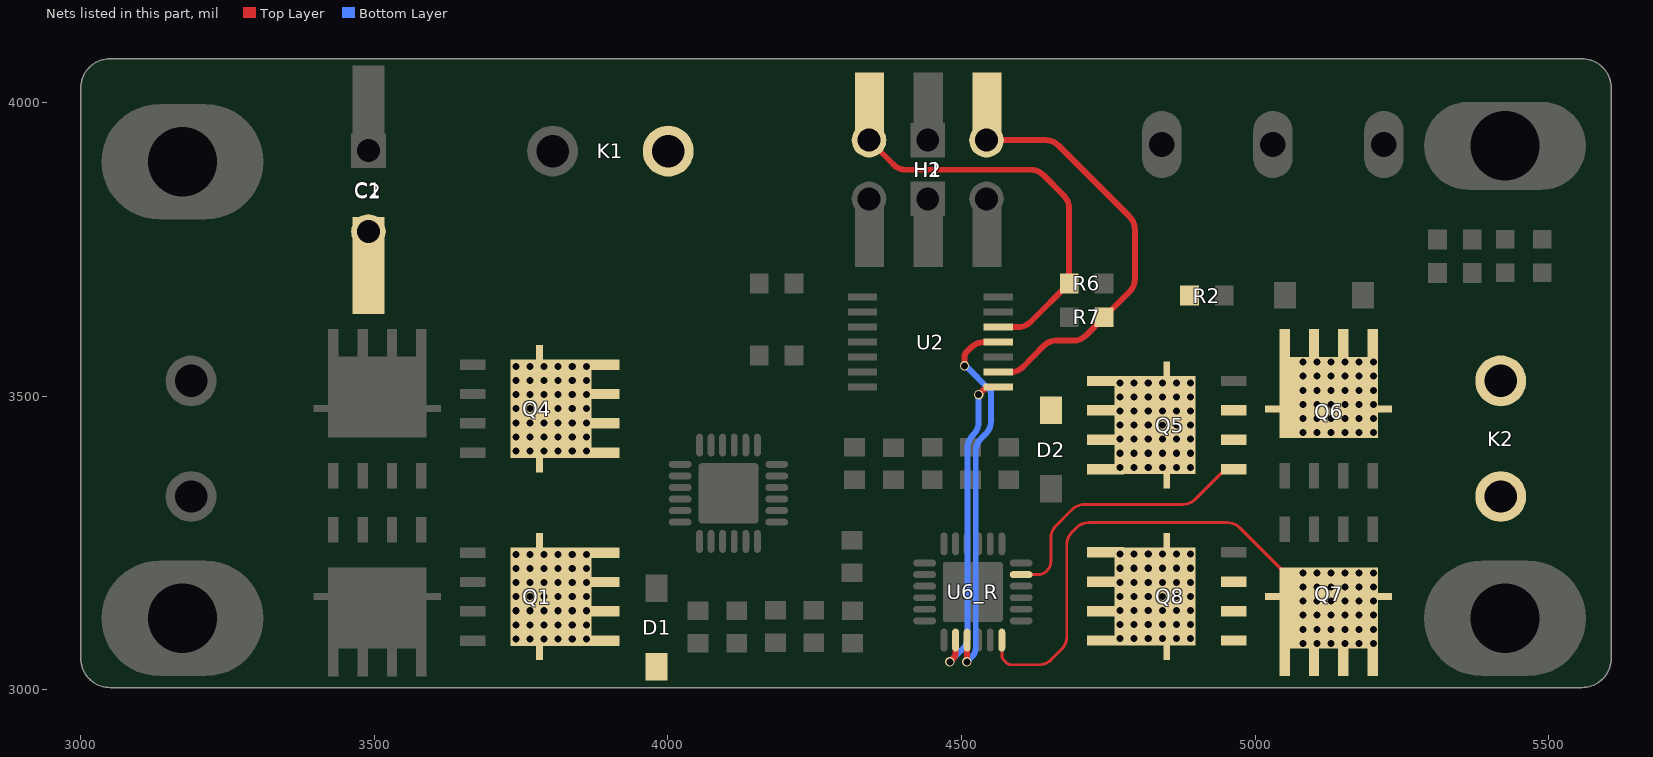
[diagram p0: the nets of this part, all layers, seen from the top]
# Altium PCB MISC49921.pcbdoc (part 2 of 2)
Units mil, origin at the board's own origin, x right, y up, seen from the top; angles counter-clockwise.
Board outline 2606.3 x 1070.87 mil, 2 copper layers (Top Layer, Bottom Layer), stack 62.206 mil thick; 46 components, 37 nets, 219 pads, 514 vias.

## Via types
v1: diameter 16, hole 12, Top Layer to Bottom Layer, 514 vias

## Nets (pads, with @x,y where several pads share a name; then routed paths per layer and width w, separated by ;. In a path a pad name is that pad's centre, name@x,y a point inside that pad or via, vN(x,y) a via of type N, cw(c..) or ccw(c..) an arc to the next point about the centre after c; other vN are vias at no path point) (continued)
R_A: K2.2 Q5.3 Q6.1 U6_R.23 | length 466.2
  Top Layer w5: U6_R.23@4601.44,3196.12 4630.24,3196.12 ccw(c4630.24,3216.12) 4644.38,3201.98 4646.13,3203.73 ccw(c4631.98,3217.87) 4651.98,3217.87 4651.98,3258.23 cw(c4681.98,3258.23) 4660.77,3279.44 4688.14,3306.81 cw(c4709.35,3285.6) 4709.35,3315.6 4876.57,3315.6 ccw(c4876.57,3345.6) 4897.79,3324.39 4946.23,3372.83 cw(c4953.3,3365.76) 4953.3,3375.76 Q5.3@4963.47,3375.76
  other v1: 5081,3437.97 5105,3437.97 5129,3437.97 5153,3437.97 5177,3437.97 5201,3437.97 5081,3461.97 5105,3461.97 5129,3461.97 5153,3461.97 5177,3461.97 5201,3461.97 5081,3485.97 5105,3485.97 5129,3485.97 5153,3485.97 5177,3485.97 5201,3485.97 5081,3509.97 5105,3509.97 5129,3509.97 5153,3509.97 5177,3509.97 5201,3509.97 5081,3533.97 5105,3533.97 5129,3533.97 5153,3533.97 5177,3533.97 5201,3533.97 5081,3557.97 5105,3557.97 5129,3557.97 5153,3557.97 5177,3557.97 5201,3557.97
R_B: K2.1 Q7.1 Q8.3 U6_R.18 | length 851.2
  Top Layer w5: U6_R.18@4568.45,3084.64 4568.45,3058.29 ccw(c4578.45,3058.29) 4571.38,3051.22 4577.06,3045.55 ccw(c4584.13,3052.62) 4584.13,3042.62 4631.59,3042.62 ccw(c4631.59,3072.62) 4652.8,3051.4 4670.24,3068.84 ccw(c4649.03,3090.06) 4679.03,3090.06 4679.03,3247.03 cw(c4709.03,3247.03) 4687.82,3268.24 4695.52,3275.94 cw(c4716.74,3254.73) 4716.74,3284.73 4952.44,3284.73 cw(c4952.44,3254.73) 4973.66,3275.94 4973.66,3275.75 5107.2,3142.21 5107.39,3142.21 ccw(c5114.47,3149.28) 5114.47,3139.28 Q7.1@5125,3139.28
  other v1: 5081,3078.96 5105,3078.96 5129,3078.96 5153,3078.96 5177,3078.96 5201,3078.96 5081,3102.96 5105,3102.96 5129,3102.96 5153,3102.96 5177,3102.96 5201,3102.96 5081,3126.96 5105,3126.96 5129,3126.96 5153,3126.96 5177,3126.96 5201,3126.96 5081,3150.96 5105,3150.96 5129,3150.96 5153,3150.96 5177,3150.96 5201,3150.96 5081,3174.96 5105,3174.96 5129,3174.96 5153,3174.96 5177,3174.96 5201,3174.96 5081,3198.96 5105,3198.96 5129,3198.96 5153,3198.96 5177,3198.96 5201,3198.96
R_DIR_IN: H1.2 H2.2 R6.2 U2.12 | length 671.2
  Top Layer w10: H2.2@4342.39,3935.88 4383.88,3894.39 ccw(c4405.1,3915.6) 4405.1,3885.6 4617.57,3885.6 cw(c4617.57,3855.6) 4638.79,3876.81 4674.21,3841.39 cw(c4653,3820.17) 4683,3820.17 4683,3692.2 R6.2@4683.13,3692.07 4617.47,3626.4 cw(c4596.26,3647.62) 4596.26,3617.62 U2.12@4561.64,3617.62
R_DIR_O: U2.11 U6_R.15 | length 657.9
  Top Layer w10: v1(4505,3551.6) 4505,3567.46 cw(c4515,3567.46) 4507.93,3574.53 4516.64,3583.24 cw(c4537.85,3562.03) 4537.85,3592.03 U2.11@4561.64,3592.03 ; v1(4509,3047.6) 4509,3084.24 U6_R.15@4509.4,3084.64
  Bottom Layer w10: v1(4505,3551.6) 4506.87,3551.6 4548,3510.47 4548,3508.6 4550,3506.6 4550,3457.03 cw(c4520,3457.03) 4541.21,3435.81 4532.79,3427.39 ccw(c4554,3406.17) 4524,3406.17 4524,3070.88 cw(c4504,3070.88) 4518.14,3056.74 v1(4509,3047.6)
R_PWM_IN: H1.6 H2.6 R7.2 U2.9 | length 709.1
  Top Layer w10: H2.6@4542.39,3935.88 4643.29,3935.88 cw(c4643.29,3905.88) 4664.51,3927.09 4786.21,3805.39 cw(c4765,3784.17) 4795,3784.17 4795,3699.34 cw(c4765,3699.34) 4786.21,3678.13 R7.2@4744.34,3636.26 ; U2.9@4561.64,3540.85 4583.15,3540.85 ccw(c4583.15,3570.85) 4604.51,3549.78 4639.9,3585.67 cw(c4661.26,3564.6) 4661.26,3594.6 4690.71,3594.6 ccw(c4690.71,3624.6) 4712.07,3603.53 R7.2@4742.45,3634.37 ; R7.2@4742.45,3634.37 R7.2@4744.34,3636.26 ; R7.2@4742.45,3634.37 R7.2@4744.34,3636.26
R_PWM_O: U2.8 U6_R.14 | length 549.1
  Top Layer w10: v1(4480,3047.6) 4486.78,3054.38 ccw(c4479.71,3061.45) 4489.71,3061.45 U6_R.14@4489.71,3084.64 ; v1(4529,3502.6) 4535.8,3509.4 cw(c4549.94,3495.26) 4549.94,3515.26 U2.8@4561.64,3515.26
  Bottom Layer w10: v1(4480,3047.6) 4501.2,3068.8 ccw(c4479.98,3090.01) 4509.98,3090.01 4509.98,3411.98 cw(c4539.98,3411.98) 4518.77,3433.19 4520.21,3434.63 ccw(c4499,3455.85) 4529,3455.85 v1(4529,3502.6)
VM: C1.1 C2.1 D1.2 D2.2 K1.1 Q1.1 Q4.1 Q5.1 Q8.1 R2.2
  other v1: 3741,3086.6 3765,3086.6 3789,3086.6 3813,3086.6 3837,3086.6 3861,3086.6 4769.79,3086.96 4793.79,3086.96 4817.79,3086.96 4841.79,3086.96 4865.79,3086.96 4889.79,3086.96 3741,3110.6 3765,3110.6 3789,3110.6 3813,3110.6 3837,3110.6 3861,3110.6 4769.79,3110.96 4793.79,3110.96 4817.79,3110.96 4841.79,3110.96 4865.79,3110.96 4889.79,3110.96 3741,3134.6 3765,3134.6 3789,3134.6 3813,3134.6 3837,3134.6 3861,3134.6 4769.79,3134.96 4793.79,3134.96 4817.79,3134.96 4841.79,3134.96 4865.79,3134.96 4889.79,3134.96 3741,3158.6 3765,3158.6 3789,3158.6 3813,3158.6 3837,3158.6 3861,3158.6 4769.79,3158.96 4793.79,3158.96 4817.79,3158.96 4841.79,3158.96 4865.79,3158.96 4889.79,3158.96 3741,3182.6 3765,3182.6 3789,3182.6 3813,3182.6 3837,3182.6 3861,3182.6 4769.79,3182.96 4793.79,3182.96 4817.79,3182.96 4841.79,3182.96 4865.79,3182.96 4889.79,3182.96 3741,3206.6 3765,3206.6 3789,3206.6 3813,3206.6 3837,3206.6 3861,3206.6 4769.79,3206.96 4793.79,3206.96 4817.79,3206.96 4841.79,3206.96 4865.79,3206.96 4889.79,3206.96 3741,3230.6 3765,3230.6 3789,3230.6 3813,3230.6 3837,3230.6 3861,3230.6 4769.79,3230.96 4793.79,3230.96 4817.79,3230.96 4841.79,3230.96 4865.79,3230.96 4889.79,3230.96 4769.79,3378.76 4793.79,3378.76 4817.79,3378.76 4841.79,3378.76 4865.79,3378.76 4889.79,3378.76 4769.79,3402.76 4793.79,3402.76 4817.79,3402.76 4841.79,3402.76 4865.79,3402.76 4889.79,3402.76 3741,3406.6 3765,3406.6 3789,3406.6 3813,3406.6 3837,3406.6 3861,3406.6 4769.79,3426.76 4793.79,3426.76 4817.79,3426.76 4841.79,3426.76 4865.79,3426.76 4889.79,3426.76 3741,3430.6 3765,3430.6 3789,3430.6 3813,3430.6 3837,3430.6 3861,3430.6 4769.79,3450.76 4793.79,3450.76 4817.79,3450.76 4841.79,3450.76 4865.79,3450.76 4889.79,3450.76 3741,3454.6 3765,3454.6 3789,3454.6 3813,3454.6 3837,3454.6 3861,3454.6 4769.79,3474.76 4793.79,3474.76 4817.79,3474.76 4841.79,3474.76 4865.79,3474.76 4889.79,3474.76 3741,3478.6 3765,3478.6 3789,3478.6 3813,3478.6 3837,3478.6 3861,3478.6 4769.79,3498.76 4793.79,3498.76 4817.79,3498.76 4841.79,3498.76 4865.79,3498.76 4889.79,3498.76 3741,3502.6 3765,3502.6 3789,3502.6 3813,3502.6 3837,3502.6 3861,3502.6 4769.79,3522.76 4793.79,3522.76 4817.79,3522.76 4841.79,3522.76 4865.79,3522.76 4889.79,3522.76 3741,3526.6 3765,3526.6 3789,3526.6 3813,3526.6 3837,3526.6 3861,3526.6 3741,3550.6 3765,3550.6 3789,3550.6 3813,3550.6 3837,3550.6 3861,3550.6
pads on no net: U6_L.9 U6_L.10 U6_L.11 U6_R.9 U6_R.10 U6_R.11

## Polygon pours and split planes (outlines as drawn)
VM on Top Layer (solid, remove dead copper, pour order 16): 3888.79,3989.85 3888.79,3714.75 4098.85,3714.75 4098.85,3989.85
VM on Bottom Layer (solid, remove dead copper, pour order 32): 3433,3830.6 3433,3739.6 3809,3739.6 3809,3830.6
VM on Bottom Layer (solid, remove dead copper, pour order 34): 3888.79,3989.85 3888.79,3730.75 4098.85,3730.75 4098.85,3989.85
VM on Top Layer (solid, remove dead copper, pour order 0): 3368.4,3830.59 3368.4,3644.33 3705.15,3644.33 3705.15,3393.67 3925.27,3393.67 3925.27,3830.59
L_A on Top Layer (solid, remove dead copper, pour order 2): 3074,3409.02 3351.58,3409.02 3406.57,3354.03 3406.57,3245.52 3416.5,3235.6 3593.14,3235.6 3643.14,3285.6 3699,3285.6 3699,3124.6 3683,3108.6 3642,3108.6 3629,3095.6 3629,3034.6 3616,3021.6 3422,3021.6 3396,3047.6 3338,3047.6 3312,3073.6 3312,3163.6 3253.77,3221.83 3074,3221.83
R_A on Top Layer (solid, remove dead copper, pour order 4): 5026,3620.6 5525.3,3620.6 5525.3,3432.07 5236.88,3432.07 5231.13,3427.56 5039.68,3427.56 5002,3389.87 5002,3363.6 4997,3358.6 4935,3358.6 4935,3491.6 4938,3494.6 4984,3494.6 4995,3505.6 4995,3589.6
R_B on Top Layer (solid, remove dead copper, pour order 6): 5525.68,3405.6 5525.68,3220.6 5345,3220.6 5287,3162.6 5287,3025.6 5284,3022.6 4967.51,3022.6 4929.57,3060.54 4929.57,3202.17 4932,3204.6 5015.23,3204.6 5033.57,3222.94 5197.46,3222.94 5231,3256.49 5231,3405.6
VM on Top Layer (solid, remove dead copper, pour order 8): 3748,3268.6 3912,3268.6 3933,3247.6 3933,3094.56 3949.86,3077.7 4014.27,3077.7 4014.27,3000 3955.6,3000 3936,3019.6 3936,3041.6 3929,3048.6 3738.55,3048.6 3726.98,3060.18 3726.98,3247.58
VM on Top Layer (solid, remove dead copper, pour order 10): 4849.3,3267.43 4726.83,3267.43 4706,3246.6 4706,3071.6 4727,3050.6 4894,3050.6 4907,3063.6 4907,3247.6 4887,3267.6 4849.47,3267.6
VM on Top Layer (solid, remove dead copper, pour order 12): 4854,3340.6 4716,3340.6 4700,3356.6 4700,3412.09 4685.35,3426.75 4628.42,3426.75 4618.42,3436.75 4618.42,3487.02 4667,3535.6 4816,3535.6 4864,3583.6 4864,3696.6 4863,3697.6 4900.87,3697.6 4907.53,3690.93 4907.53,3542.13 4899,3533.6 4899,3366.6 4880,3366.6
GND on Top Layer (solid, remove dead copper, pour order 18): 3050,4074.6 ccw(c3050,4024.6) 3000,4024.6 3000,3053.73 ccw(c3050,3053.73) 3050,3003.73 5556.3,3003.73 ccw(c5556.3,3053.73) 5606.3,3053.73 5606.3,4024.6 ccw(c5556.3,4024.6) 5556.3,4074.6
VM on Bottom Layer (solid, remove dead copper, pour order 20): 3726.98,3075.6 3928,3075.6 3928,3830.59 3706,3830.59 3706,3268.55 3726.98,3247.58
VM on Bottom Layer (solid, remove dead copper, pour order 22): 4909,3074.6 4712,3074.6 4712,3534.6 4713,3535.6 4646.81,3601.79 4038.17,3601.79 3928.98,3492.6 3899,3492.6 3899,3793.6 3896,3796.6 4815,3796.6 4909,3702.6
GND on Bottom Layer (solid, remove dead copper, pour order 36): 3050,4074.6 ccw(c3050,4024.6) 3000,4024.6 3000,3053.73 ccw(c3050,3053.73) 3050,3003.73 5556.3,3003.73 ccw(c5556.3,3053.73) 5606.3,3053.73 5606.3,4024.6 ccw(c5556.3,4024.6) 5556.3,4074.6
R_A on Bottom Layer (solid, remove dead copper, pour order 30): 5071.68,3616.6 5526.3,3616.6 5526.3,3432.07 5236.47,3432.07 5231.96,3427.56 5071.68,3427.56
R_B on Bottom Layer (solid, remove dead copper, pour order 28): 5526.68,3405.6 5526.68,3220.6 5345,3220.6 5287,3162.6 5287,3069.6 5071.57,3069.6 5071.57,3222.94 5197.46,3222.94 5231,3256.49 5231,3405.6
L_B on Bottom Layer (solid, remove dead copper, pour order 26): 3557.15,3626.6 3074,3626.6 3074,3430.75 3557.15,3430.75
L_A on Bottom Layer (solid, remove dead copper, pour order 24): 3074,3409.02 3351.58,3409.02 3406.57,3354.03 3406.57,3245.52 3416.5,3235.6 3558.14,3235.6 3558.14,3069.6 3316,3069.6 3312,3073.6 3312,3163.6 3253.77,3221.83 3074,3221.83
L_B on Top Layer (solid, remove dead copper, pour order 14): 3695,3626.6 3074,3626.6 3074,3430.75 3695,3430.75

## Keep-outs
Board Outline Layer:
  the board outline again, w10

## Other copper
Top Layer:
  region net AVDD_L: 4291.01,3149.46 4299.05,3155.56 4302.65,3153.29 4306.57,3151.62 4310.71,3150.6 4314.96,3150.26 4296.31,3133.55 4295.97,3137.8 4294.95,3141.93 4293.28,3145.86 4291.01,3149.46
  region net $1N3247: 4159.98,3146.55 4164.5,3156.17 4168.1,3153.9 4172.02,3152.23 4176.16,3151.21 4180.41,3150.87 4165.28,3130.64 4164.94,3134.89 4163.92,3139.02 4162.25,3142.95 4159.98,3146.55
  region net $1N3253: 4153.73,3095.13 4169.84,3107.3 4174.29,3103.88 4179.11,3101.01 4184.23,3098.73 4189.6,3097.08 4195.12,3096.08 4200.72,3095.75 4165.28,3064.25 4164.95,3069.85 4163.95,3075.37 4162.3,3080.73 4160.03,3085.86 4157.16,3090.68 4153.73,3095.13
  region net AVDD_R: 4340.9,3343.77 4333.55,3336.98 4329.94,3339.26 4326.02,3340.93 4321.88,3341.95 4317.64,3342.29 4335.6,3359.68 4335.94,3355.43 4336.96,3351.3 4338.63,3347.37 4340.9,3343.77
  region net $1N3253: 4048.79,3165.26 4058.79,3165.26 4059.11,3161.8 4060.06,3158.46 4061.62,3155.36 4063.72,3152.59 4066.29,3150.26 4041.29,3150.26 4043.86,3152.59 4045.96,3155.36 4047.51,3158.46 4048.47,3161.8 4048.79,3165.26
  region net $1N3253: 4099.04,3144.51 4099.04,3124.51 4091.37,3124.15 4083.77,3123.06 4076.3,3121.26 4069.04,3118.76 4069.04,3150.26 4076.3,3147.76 4083.77,3145.96 4091.37,3144.87 4099.04,3144.51
  region net $1N4036: 4573.45,3337.84 4563.45,3337.84 4563.25,3340.1 4562.65,3342.29 4581.45,3342.29 4579.09,3341.99 4576.87,3341.1 4574.95,3339.69 4573.45,3337.84
  region net $1N4036: 4628.08,3362.44 4628.08,3342.44 4613.08,3342.4 4598.08,3342.29 4598.08,3373.78 4602.38,3370.42 4607.06,3367.6 4612.04,3365.37 4617.26,3363.75 4622.63,3362.77 4628.08,3362.44
  region net $1N4036: 4532.65,3348.04 4532.65,3368.04 4540.32,3368.4 4547.92,3369.49 4555.39,3371.29 4562.65,3373.78 4562.65,3342.29 4555.39,3344.79 4547.92,3346.59 4540.32,3347.67 4532.65,3348.04
  region net $1N3022: 4225.1,3092.87 4231.06,3101.05 4234.67,3098.78 4238.59,3097.11 4242.73,3096.09 4246.97,3095.75 4230.4,3076.96 4230.06,3081.21 4229.04,3085.35 4227.38,3089.27 4225.1,3092.87
  region net $1N3253: 4152.09,3125.06 4140.7,3108.16 4135.98,3111.32 4130.94,3113.96 4125.65,3116.04 4120.17,3117.55 4114.56,3118.46 4108.88,3118.76 4134.86,3150.26 4138.27,3143.38 4142.3,3136.86 4146.92,3130.73 4152.09,3125.06
  region net $1N3253: 4069.43,3124.51 4069.43,3144.51 4077.1,3144.87 4084.7,3145.96 4092.17,3147.76 4099.43,3150.26 4099.43,3118.76 4092.17,3121.26 4084.7,3123.06 4077.1,3124.15 4069.43,3124.51
  region net $1N4031: 4395.61,3327.08 4383.29,3327.08 4379.89,3332.38 4375.91,3337.27 4371.4,3341.68 4396.4,3341.68 4394.59,3339.65 4393.38,3337.21 4392.87,3334.55 4393.09,3331.84 4394.03,3329.28 4395.61,3327.08
  region net $1N4029: 4406.81,3396.6 4397.77,3391.49 4394.16,3393.77 4390.24,3395.44 4386.11,3396.46 4381.86,3396.8 4401.5,3412.51 4401.85,3408.26 4402.87,3404.12 4404.53,3400.2 4406.81,3396.6
  region net $1N4036: 4480.97,3368.16 4493.03,3384.39 4497.75,3381.23 4502.79,3378.59 4508.08,3376.51 4513.56,3375 4519.17,3374.09 4524.85,3373.78 4497.53,3342.29 4495.14,3348 4492.27,3353.48 4488.93,3358.69 4485.16,3363.6 4480.97,3368.16
  region net $1N4036: 4562.96,3368.04 4562.96,3348.04 4555.29,3347.67 4547.69,3346.59 4540.22,3344.79 4532.96,3342.29 4532.96,3373.78 4540.22,3371.29 4547.69,3369.49 4555.29,3368.4 4562.96,3368.04
  region net $1N4034: 4473.14,3342.09 4464.1,3336.98 4460.5,3339.26 4456.58,3340.93 4452.44,3341.95 4448.19,3342.29 4467.84,3358 4468.18,3353.75 4469.2,3349.61 4470.87,3345.69 4473.14,3342.09
  region net $1N4036: 4479.39,3398.03 4463.28,3385.86 4458.84,3389.28 4454.02,3392.15 4448.89,3394.42 4443.53,3396.07 4438.01,3397.07 4432.41,3397.41 4467.84,3428.9 4468.17,3423.3 4469.17,3417.78 4470.82,3412.42 4473.1,3407.29 4475.97,3402.47 4479.39,3398.03
  region net $1N3253: 4010.11,3157.82 4000.89,3138.75 3996.17,3141.92 3991.13,3144.55 3985.84,3146.64 3980.36,3148.14 3974.75,3149.06 3969.07,3149.36 3999.51,3189.64 3999.81,3183.96 4000.72,3178.35 4002.23,3172.87 4004.31,3167.58 4006.95,3162.54 4010.11,3157.82
  region net $1N4036: 4603.18,3342.44 4603.18,3362.44 4613.25,3362.81 4623.27,3363.91 4633.18,3365.74 4633.18,3327.44 4629.95,3331.2 4626.24,3334.51 4622.14,3337.29 4617.7,3339.51 4613,3341.13 4608.14,3342.11 4603.18,3342.44
  region net $1N595: 5394.75,3704.97 5394.75,3714.97 5398.21,3715.29 5401.55,3716.25 5404.65,3717.8 5407.42,3719.9 5409.75,3722.47 5409.75,3697.47 5407.42,3700.05 5404.65,3702.15 5401.55,3703.7 5398.21,3704.65
  region net PWR_EN: 5279.46,3761.89 5279.46,3771.89 5282.92,3772.21 5286.26,3773.16 5289.37,3774.72 5292.13,3776.82 5294.46,3779.39 5294.46,3754.39 5292.13,3756.96 5289.37,3759.06 5286.26,3760.61 5282.92,3761.57 5279.46,3761.89
  region net $1N440: 5400.54,3771.89 5400.54,3761.89 5397.08,3761.57 5393.74,3760.61 5390.63,3759.06 5387.87,3756.96 5385.54,3754.39 5385.54,3779.39 5387.87,3776.82 5390.63,3774.72 5393.74,3773.16 5397.08,3772.21 5400.54,3771.89
  region net 3V6: 4978.18,3676.08 4978.18,3666.08 4974.73,3665.76 4971.39,3664.81 4968.28,3663.26 4965.51,3661.16 4963.18,3658.58 4963.18,3683.58 4965.51,3681.01 4968.28,3678.91 4971.39,3677.36 4974.73,3676.41 4978.18,3676.08
  region net 3V6: 5279.46,3704.87 5279.46,3714.87 5282.92,3715.19 5286.26,3716.15 5289.37,3717.7 5292.13,3719.8 5294.46,3722.37 5294.46,3697.37 5292.13,3699.95 5289.37,3702.05 5286.26,3703.6 5282.92,3704.55 5279.46,3704.87
  region net $1N595: 5400.54,3714.97 5400.54,3704.97 5397.08,3704.65 5393.74,3703.7 5390.63,3702.15 5387.87,3700.05 5385.54,3697.47 5385.54,3722.47 5387.87,3719.9 5390.63,3717.8 5393.74,3716.25 5397.08,3715.29 5400.54,3714.97
  region net L_DIR_IN: 4235.84,3677.96 4229.9,3669.76 4226.3,3672.03 4222.38,3673.7 4218.24,3674.72 4213.99,3675.06 4230.54,3693.87 4230.88,3689.62 4231.9,3685.48 4233.57,3681.56 4235.84,3677.96
  region net R_DIR_IN: 4667.89,3669.76 4661.96,3677.96 4664.23,3681.56 4665.9,3685.48 4666.92,3689.62 4667.26,3693.87 4683.8,3675.06 4679.56,3674.72 4675.42,3673.7 4671.5,3672.03 4667.89,3669.76
  region net R_DIR_IN: 4678,3724.08 4688,3724.08 4688.32,3720.62 4689.28,3717.28 4690.83,3714.17 4692.93,3711.41 4695.5,3709.08 4670.5,3709.08 4673.07,3711.41 4675.17,3714.17 4676.72,3717.28 4677.68,3720.62 4678,3724.08
  region net GND: 4726.94,3664.03 4713.93,3679.3 4717.57,3683.45 4720.66,3688.03 4723.14,3692.96 4724.97,3698.17 4726.13,3703.57 4726.58,3709.08 4758.33,3675.06 4752.69,3674.74 4747.12,3673.79 4741.69,3672.22 4736.48,3670.05 4731.54,3667.31 4726.94,3664.03
  region net R_PWM_IN: 4727.39,3611.95 4721.39,3620.1 4723.62,3623.73 4725.25,3627.66 4726.24,3631.8 4726.58,3636.05 4743.26,3617.36 4739.01,3617.01 4734.88,3615.97 4730.97,3614.27 4727.39,3611.95
  region net R_PWM_IN: 4757.69,3656.68 4763.63,3648.47 4761.36,3644.87 4759.69,3640.95 4758.67,3636.81 4758.33,3632.56 4741.78,3651.37 4746.03,3651.72 4750.17,3652.74 4754.09,3654.4 4757.69,3656.68
  region net GND: 4697.84,3663.22 4710.85,3647.94 4707.35,3643.59 4704.41,3638.84 4702.07,3633.76 4700.38,3628.43 4699.35,3622.94 4699.01,3617.36 4667.26,3651.37 4672.84,3651.72 4678.33,3652.75 4683.66,3654.44 4688.74,3656.77 4693.49,3659.71 4697.84,3663.22
  region net PWR_EN: 5035.01,3858.81 5025.01,3858.81 5024.91,3861.08 5024.61,3863.36 5024.1,3865.6 5023.34,3867.71 5022.32,3869.66 5021.02,3871.36 5019.42,3872.77 5017.51,3873.81 5042.51,3873.81 5040.59,3872.77 5038.99,3871.36 5037.69,3869.66 5036.67,3867.71 5035.91,3865.6 5035.4,3863.36 5035.1,3861.08
  region net 3V6: 5016.67,3666.08 5016.67,3676.08 5020.13,3676.41 5023.47,3677.36 5026.57,3678.91 5029.34,3681.01 5031.67,3683.58 5031.67,3658.58 5029.34,3661.16 5026.57,3663.26 5023.47,3664.81 5020.13,3665.76 5016.67,3666.08
  region net 3V6: 5071.24,3699.42 5074.37,3688.41 5072.1,3684.81 5070.43,3680.89 5069.41,3676.75 5069.07,3672.5 5055.33,3694.12 5059.58,3694.46 5063.72,3695.48 5067.64,3697.14 5071.24,3699.42
  region net $1N440: 5394.75,3761.89 5394.75,3771.89 5398.21,3772.21 5401.55,3773.16 5404.65,3774.72 5407.42,3776.82 5409.75,3779.39 5409.75,3754.39 5407.42,3756.96 5404.65,3759.06 5401.55,3760.61 5398.21,3761.57
  region net R_DIR_IN: 4374.43,3910.91 4367.36,3903.84 4365.72,3905.34 4364.15,3906.51 4362.65,3907.36 4361.19,3907.94 4359.76,3908.29 4358.34,3908.43 4355.45,3908.25 4349.01,3906.99 4345.18,3906.48 4343.04,3906.38 4340.75,3906.43 4371.84,3937.52 4371.89,3935.23 4371.79,3933.1 4371.28,3929.26 4370.03,3922.82 4369.84,3919.93 4369.98,3918.51 4370.33,3917.08 4370.91,3915.62 4371.76,3914.12 4372.93,3912.55
  region net R_PWM_IN: 4582.71,3940.88 4582.71,3930.88 4580.48,3930.78 4578.55,3930.5 4576.88,3930.04 4575.44,3929.42 4574.18,3928.65 4573.08,3927.75 4571.16,3925.57 4567.5,3920.13 4565.15,3917.06 4563.71,3915.48 4562.06,3913.89 4562.06,3957.87 4563.71,3956.28 4565.15,3954.7 4567.5,3951.63 4571.16,3946.19 4573.08,3944.02 4574.18,3943.11 4575.44,3942.34 4576.88,3941.72 4578.55,3941.26 4580.48,3940.98
  region net L_DIR_IN: 4322.49,3715.02 4312.85,3719.53 4315.13,3723.13 4316.8,3727.05 4317.82,3731.19 4318.16,3735.44 4338.4,3720.33 4334.16,3719.98 4330.02,3718.96 4326.1,3717.3 4322.49,3715.02
  region net L_PWM_IN: 4518.49,3715.02 4512.85,3723.53 4515.13,3727.13 4516.8,3731.05 4517.82,3735.19 4518.16,3739.44 4534.4,3720.33 4530.16,3719.98 4526.02,3718.96 4522.1,3717.3 4518.49,3715.02
  region net GL1_L: 3997.16,3381.31 3997.16,3386.31 4000.97,3387.56 4004.66,3389.13 4004.66,3378.48 4000.97,3380.05 3997.16,3381.31
  region net L_B: 4040.38,3414.06 4040.38,3419.06 4042.54,3419.31 4044.58,3420.05 4046.39,3421.23 4047.88,3422.81 4047.88,3410.31 4046.39,3411.88 4044.58,3413.07 4042.54,3413.81 4040.38,3414.06
  region net GH1_L: 4070.97,3436.99 4075.97,3436.99 4077.24,3434.75 4078.8,3432.7 4068.14,3432.7 4069.7,3434.75 4070.97,3436.99
  region net AVDD_L: 4208.51,3388.81 4208.51,3378.81 4203.63,3378.58 4198.79,3377.9 4198.79,3389.71 4203.63,3389.03 4208.51,3388.81
  region net GL2_R: 4625.08,3178.94 4625.08,3173.94 4621.27,3172.69 4617.58,3171.12 4617.58,3181.77 4621.27,3180.2 4625.08,3178.94
  region net GL1_R: 4624.87,3120.1 4625.28,3115.1 4621.45,3113.84 4617.78,3112.17 4617.37,3122.82 4621.08,3121.35 4624.87,3120.1
  region net PWR_EN: 4455,3078.6 4455,3088.6 4457.53,3088.95 4459.86,3089.97 4461.84,3091.59 4463.29,3093.69 4464.13,3096.1 4464.13,3071.1 4463.29,3073.51 4461.84,3075.61 4459.86,3077.23 4457.53,3078.25
  region net AVDD_R: 4408.45,3112.39 4408.45,3122.39 4415.96,3122.62 4423.45,3123.3 4423.45,3111.49 4415.96,3112.17 4408.45,3112.39
  region net L_DIR_IN: 4291.32,3638.21 4291.32,3648.21 4298.83,3648.46 4306.32,3649.21 4306.32,3637.21 4298.83,3637.96 4291.32,3638.21
  region net L_DIR_O: 4291.32,3612.62 4291.32,3622.62 4298.83,3622.87 4306.32,3623.62 4306.32,3611.62 4298.83,3612.37 4291.32,3612.62
  region net L_PWM_IN: 4291.32,3561.44 4291.32,3571.44 4298.83,3571.69 4306.32,3572.44 4306.32,3560.44 4298.83,3561.19 4291.32,3561.44
  region net L_PWM_IN: 4366.93,3577.67 4370.23,3567.59 4365.4,3565.6 4360.75,3563.21 4356.32,3560.44 4356.32,3572.44 4360.14,3573.55 4363.72,3575.31 4366.93,3577.67
  region net L_PWM_O: 4291.32,3535.85 4291.32,3545.85 4298.83,3546.1 4306.32,3546.85 4306.32,3534.85 4298.83,3535.6 4291.32,3535.85
  region net R_PWM_O: 4539.33,3505.86 4532.26,3512.93 4534.44,3515.44 4536.24,3518.24 4537.64,3521.26 4565.45,3509.26 4556.65,3508.88 4547.93,3507.74 4539.33,3505.86
  region net R_PWM_IN: 4598.75,3551.31 4601.87,3541.27 4596.93,3539.58 4592.17,3537.43 4587.64,3534.85 4587.64,3546.85 4591.61,3547.6 4595.36,3549.11 4598.75,3551.31
  region net R_DIR_O: 4522.67,3581.88 4522.67,3593.56 4527.8,3594.52 4532.81,3596.01 4537.64,3598.03 4537.64,3586.03 4533.66,3586.09 4529.75,3585.41 4526.04,3583.99 4522.67,3581.88
  region net R_DIR_IN: 4596.26,3622.62 4596.26,3612.62 4591.92,3612.36 4587.64,3611.62 4587.64,3623.62 4591.92,3622.87 4596.26,3622.62
  region net D3V3: 4537.62,3663.8 4537.62,3673.8 4537.63,3674.3 4537.64,3674.8 4537.64,3662.8 4537.63,3663.3 4537.62,3663.8
  region net L_A: 3664.81,3249.96 3669.81,3249.96 3670.06,3247.81 3670.8,3245.77 3671.99,3243.95 3673.56,3242.46 3661.06,3242.46 3662.64,3243.95 3663.82,3245.77 3664.56,3247.81 3664.81,3249.96
  region net GH2_L: 3687.97,3095.11 3691.62,3091.68 3690.17,3089.24 3689.27,3086.55 3688.97,3083.73 3680.02,3092.46 3682.84,3092.76 3685.53,3093.66 3687.97,3095.11
  region net GL2_L: 3436.94,3297.08 3441.51,3294.57 3440.06,3292.13 3439.16,3289.44 3438.86,3286.62 3428.99,3294.43 3431.81,3294.73 3434.5,3295.63 3436.94,3297.08
  region net L_B: 3591.31,3429.82 3587.33,3426.74 3584.89,3428.19 3582.2,3429.08 3579.37,3429.39 3588.66,3437.78 3588.97,3434.96 3589.86,3432.26 3591.31,3429.82
  region net L_B: 3522.9,3491.17 3532.68,3488.45 3534.67,3486.77 3536.91,3485.44 3539.34,3484.51 3526.84,3484.51 3525.91,3486.94 3524.58,3489.18 3522.9,3491.17
  region net L_B: 3555.1,3466.03 3545.32,3468.75 3543.33,3470.43 3541.09,3471.76 3538.66,3472.7 3551.16,3472.7 3552.09,3470.26 3553.42,3468.02 3555.1,3466.03
  region net GH1_L: 3691.62,3396.52 3688.97,3392.09 3686.53,3393.54 3683.84,3394.44 3681.02,3394.74 3688.97,3404.47 3689.27,3401.65 3690.17,3398.96 3691.62,3396.52
  region net R_A: 4941.18,3364.25 4939.17,3369.3 4940.62,3371.74 4941.52,3374.44 4941.82,3377.26 4949.14,3366.9 4946.32,3366.6 4943.62,3365.7 4941.18,3364.25
  region net GH2_R: 4943.19,3514.25 4939.17,3517.3 4940.62,3519.74 4941.52,3522.44 4941.82,3525.26 4951.14,3516.9 4948.32,3516.6 4945.62,3515.7 4943.19,3514.25
  region net GL2_R: 5192.78,3339.84 5188.49,3342.63 5189.94,3345.07 5190.84,3347.76 5191.14,3350.58 5200.73,3342.49 5197.91,3342.19 5195.22,3341.29 5192.78,3339.84
  region net GH1_R: 4939.17,3239.9 4940.66,3245.47 4943.1,3244.02 4945.8,3243.13 4948.62,3242.82 4941.82,3231.94 4941.52,3234.76 4940.62,3237.46 4939.17,3239.9
  region net R_DIR_O: 4500,3562.53 4510,3562.53 4509.92,3559.52 4510.18,3558.2 4510.96,3556.93 4499.04,3556.93 4499.82,3558.2 4500.08,3559.52
  region net PWR_EN: 4465.93,3088.6 4465.93,3078.6 4462.92,3078.68 4461.6,3078.42 4460.33,3077.64 4460.33,3089.56 4461.6,3088.78 4462.92,3088.52
  region net GND: 3580.93,3408.6 3580.93,3398.6 3577.92,3398.68 3576.6,3398.42 3575.33,3397.64 3575.33,3409.56 3576.6,3408.78 3577.92,3408.52
  region net L_B: 3520.48,3493.59 3524.85,3496.29 3525.9,3495.43 3527.16,3494.63 3529.61,3493.14 3517.99,3490.46 3518.69,3491.23 3519.69,3492.09 3520.47,3492.92 3520.6,3493.28
  region net L_B: 3534.69,3486.45 3535.63,3478.44 3534.96,3478.98 3534.18,3479.43 3532.38,3480.01 3530.52,3480.09 3529.64,3479.92 3528.86,3479.59 3531.54,3491.21 3533.03,3488.76 3533.83,3487.5
  region net L_B: 3540.84,3473.23 3548.85,3472.29 3549.9,3471.43 3551.16,3470.63 3553.61,3469.14 3541.99,3466.46 3542.32,3467.24 3542.49,3468.12 3542.41,3469.98 3541.83,3471.78 3541.38,3472.56
  region net L_B: 3558.69,3462.45 3559.63,3454.44 3558.96,3454.98 3558.18,3455.43 3556.38,3456.01 3554.52,3456.09 3553.64,3455.92 3552.86,3455.59 3555.54,3467.21 3557.03,3464.76 3557.83,3463.5
  region net GND: 4981.07,3728.6 4981.07,3738.6 4984.08,3738.52 4985.4,3738.78 4986.67,3739.56 4986.67,3727.64 4985.4,3728.42 4984.08,3728.68
  region net L_DIR_IN: 4270.95,3663.13 4270.63,3659.69 4269.69,3656.37 4268.15,3653.28 4266.07,3650.53 4263.53,3648.21 4275.95,3643.21 4290.95,3648.21 4288.15,3649.69 4285.7,3651.7 4283.68,3654.15 4282.19,3656.94 4281.26,3659.97 4280.95,3663.13 4270.95,3663.13
  region net PWR_EN: 5025.01,3801.89 5024.72,3796.54 5023.86,3791.25 5022.44,3786.08 5020.47,3781.09 5017.99,3776.34 5015.01,3771.89 5029.26,3766.89 5045.01,3771.89 5042.02,3776.34 5039.54,3781.09 5037.57,3786.08 5036.15,3791.25 5035.29,3796.54 5035.01,3801.89 5025.01,3801.89
  text "2026.4" at 5332,4012.6 h45
Bottom Layer:
  region net 3V6: 4846.02,3858.81 4836.02,3858.81 4835.93,3861.08 4835.63,3863.36 4835.12,3865.6 4834.36,3867.71 4833.34,3869.66 4832.04,3871.36 4830.44,3872.77 4828.52,3873.81 4853.52,3873.81 4851.61,3872.77 4850.01,3871.36 4848.71,3869.66 4847.69,3867.71 4846.93,3865.6 4846.42,3863.36 4846.12,3861.08
  region net D3V3: 4399.14,3191.6 4399.14,3201.6 4402.12,3201.53 4403.42,3201.79 4404.67,3202.56 4404.67,3190.64 4403.42,3191.41 4402.12,3191.68
  region net D3V3: 4338.27,3260.4 4331.2,3253.33 4329.12,3255.53 4328.01,3256.27 4326.55,3256.61 4334.99,3265.05 4335.33,3263.59 4336.07,3262.48
  region net D3V3: 4222.93,3310.08 4222.93,3300.08 4219.92,3300.16 4218.6,3299.9 4217.33,3299.11 4217.33,3311.04 4218.6,3310.25 4219.92,3309.99
  region net D3V3: 4285.73,3268.8 4292.8,3275.87 4294.88,3273.67 4295.99,3272.93 4297.45,3272.59 4289.01,3264.16 4288.67,3265.61 4287.93,3266.72
  region net D3V3: 4307.93,3269.6 4307.93,3259.6 4304.92,3259.68 4303.6,3259.42 4302.33,3258.64 4302.33,3270.56 4303.6,3269.78 4304.92,3269.52
  region net D3V3: 4386.8,3505.33 4379.73,3512.4 4381.93,3514.48 4382.67,3515.59 4383.01,3517.05 4391.45,3508.61 4389.99,3508.27 4388.88,3507.53
  region net R_DIR_O: 4516.45,3549.09 4510.78,3540.62 4509.65,3541.81 4508.57,3542.83 4507.37,3543.51 4506.67,3543.66 4505.88,3543.65 4512.8,3553.36 4513.36,3551.93 4514.18,3550.98 4515.23,3550.15
  region net R_PWM_O: 4484.2,3058.87 4491.27,3051.8 4489.07,3049.72 4488.33,3048.61 4487.99,3047.16 4479.55,3055.59 4481.01,3055.93 4482.12,3056.67
  region net PWR_EN: 4444.07,3078.6 4444.07,3088.6 4447.08,3088.52 4448.4,3088.78 4449.67,3089.56 4449.67,3077.64 4448.4,3078.42 4447.08,3078.68
  region net PWR_EN: 4174,3405.67 4164,3405.67 4164.08,3408.68 4163.82,3410 4163.04,3411.27 4174.96,3411.27 4174.18,3410 4173.92,3408.68
  region net 3V6: 4928,3695.53 4938,3695.53 4937.92,3692.52 4938.18,3691.2 4938.96,3689.93 4927.04,3689.93 4927.82,3691.2 4928.08,3692.52

## Silkscreen, mask and mechanical layers (free items; w line width, h text height)
Top Silkscreen Layer:
  text "R_DIR" at 4123,3909.6 h60
  text "R_PWM" at 4605.89,3909.6 h60
  text "L_DIR" at 4123,3781.6 h60
  text "L_PWM" at 4605.89,3781.6 h60
  text "GND" at 4415,3688.6 h40
  text "-" at 3754,3584.6 h200
  text "+" at 3953,3584.6 h200
Bottom Silkscreen Layer:
  text "GND" at 4252,3976.6 h60
  text "R_DIR" at 3883,3909.6 h60
  text "R_PWM" at 4365.89,3909.6 h60
  text "L_DIR" at 3883,3782.06 h60
  text "L_PWM" at 4365.89,3782.06 h60
  text "-" at 3854,3716.6 h200
  text "+" at 4048,3712.6 h200
Top Solder Mask Layer:
  text "2026.4" at 5332,4012.6 h45